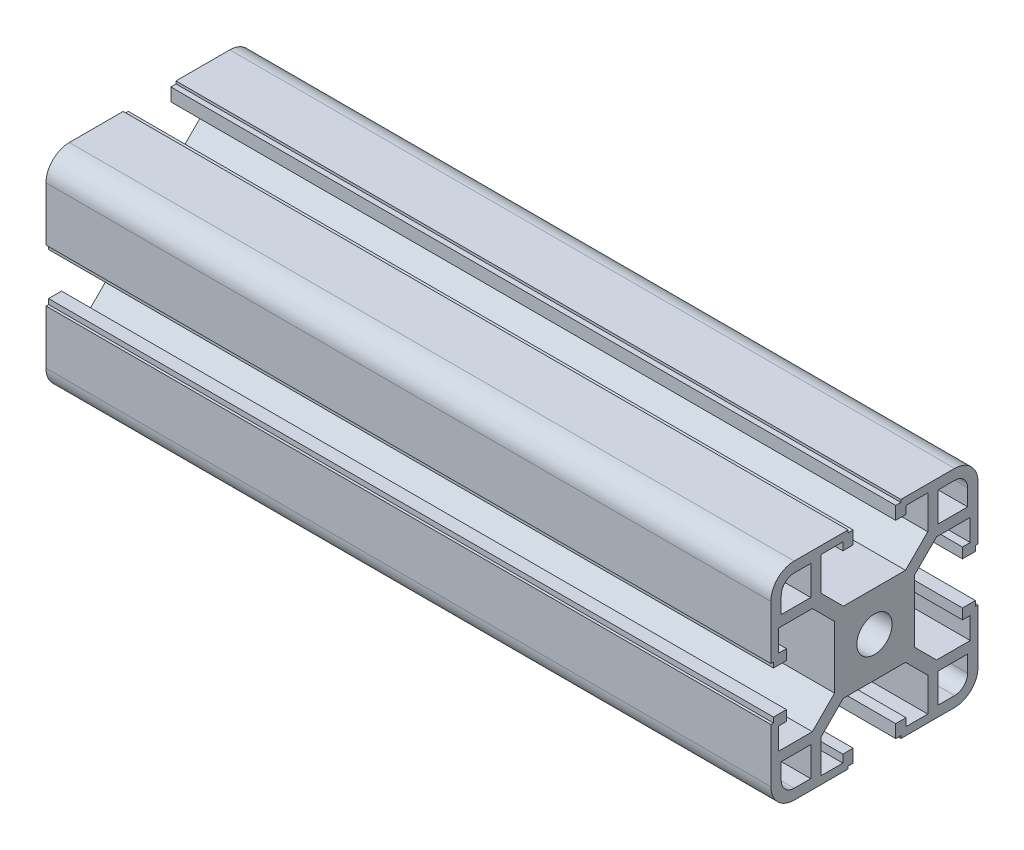
SolidWorks part; units mm, degrees
ref_plane "Front Plane" through (0, 0, 0) normal (0, 0, 1) x (1, 0, 0)
ref_plane "Top Plane" through (0, 0, 0) normal (0, 1, 0) x (1, 0, 0)
ref_plane "Right Plane" through (0, 0, 0) normal (1, 0, 0) x (0, 0, -1)
sketch "草图1" plane through (0, 0, 0) normal (0, 0, 1) x (1, 0, 0)
  line L0 (-984.975, 0) -> (-844.975, 0)
  dimension "D1" = 140
other "Aluminium profile 40 X 40B X R4.5(1)"
ref_plane "Plane1" through (-984.975, 0, 0) normal (1, 0, 0) x (0, 1, 0)
sketch "Sketch1" plane through (-984.975, 0, 0) normal (1, 0, 0) x (0, 1, 0)
  line L0 (-5.1, 20) -> (-5.1, 19.5)
  line L1 (-5.1, 19.5) -> (-4.1, 19.5)
  line L2 (-4.1, 19.5) -> (-4.1, 17)
  line L3 (-6.1, 18.5) -> (-10.3, 18.5)
  line L4 (-15.5, -20) -> (-5.1, -20)
  line L5 (-20, -15.5) -> (-20, -5.1)
  line L6 (15.5, 20) -> (5.1, 20)
  line L7 (20, 15.5) -> (20, 5.1)
  line L8 (0, 14.8756) -> (0, 0) construction
  line L9 (0, 0) -> (14.1675, 0) construction
  line L10 (-10.3, 18.5) -> (-10.3, 12)
  line L11 (-10.3, 12) -> (-6, 7.7)
  line L12 (-6, 7.7) -> (6, 7.7)
  line L13 (10.3, 12) -> (6, 7.7)
  line L14 (10.3, 18.5) -> (10.3, 12)
  line L15 (6.1, 18.5) -> (10.3, 18.5)
  line L16 (4.1, 19.5) -> (4.1, 17)
  line L17 (5.1, 19.5) -> (4.1, 19.5)
  line L18 (5.1, 20) -> (5.1, 19.5)
  line L19 (-5.1, 20) -> (-15.5, 20)
  line L20 (20, 5.1) -> (19.5, 5.1)
  line L21 (12.3, 18) -> (15.5, 18)
  line L22 (12.3, 18) -> (12.3, 12.3)
  line L23 (12.3, 12.3) -> (18, 12.3)
  line L24 (18, 15.5) -> (18, 12.3)
  line L25 (19.5, 5.1) -> (19.5, 4.1)
  line L26 (19.5, 4.1) -> (17, 4.1)
  line L27 (17, 6.1) -> (17, 4.1)
  line L28 (18.5, 6.1) -> (17, 6.1)
  line L29 (18.5, 6.1) -> (18.5, 10.3)
  line L30 (18.5, 10.3) -> (12, 10.3)
  line L31 (12, 10.3) -> (7.7, 6)
  line L32 (7.7, 6) -> (7.7, -6)
  line L33 (12, -10.3) -> (7.7, -6)
  line L34 (18.5, -10.3) -> (12, -10.3)
  line L35 (18.5, -6.1) -> (18.5, -10.3)
  line L36 (18.5, -6.1) -> (17, -6.1)
  line L37 (17, -4.1) -> (17, -6.1)
  line L38 (19.5, -4.1) -> (17, -4.1)
  line L39 (19.5, -5.1) -> (19.5, -4.1)
  line L40 (20, -5.1) -> (19.5, -5.1)
  line L41 (5.1, -20) -> (5.1, -19.5)
  line L42 (5.1, -19.5) -> (4.1, -19.5)
  line L43 (4.1, -19.5) -> (4.1, -17)
  line L44 (6.1, -17) -> (4.1, -17)
  line L45 (6.1, -18.5) -> (6.1, -17)
  line L46 (6.1, -18.5) -> (10.3, -18.5)
  line L47 (10.3, -18.5) -> (10.3, -12)
  line L48 (10.3, -12) -> (6, -7.7)
  line L49 (6, -7.7) -> (-6, -7.7)
  line L50 (-10.3, -12) -> (-6, -7.7)
  line L51 (-10.3, -18.5) -> (-10.3, -12)
  line L52 (-6.1, -18.5) -> (-10.3, -18.5)
  line L53 (-6.1, -18.5) -> (-6.1, -17)
  line L54 (-4.1, -17) -> (-6.1, -17)
  line L55 (-4.1, -19.5) -> (-4.1, -17)
  line L56 (-5.1, -19.5) -> (-4.1, -19.5)
  line L57 (-5.1, -20) -> (-5.1, -19.5)
  line L58 (-20, -5.1) -> (-19.5, -5.1)
  line L59 (5.1, -20) -> (15.5, -20)
  line L60 (-20, 5.1) -> (-20, 15.5)
  line L61 (-19.5, -5.1) -> (-19.5, -4.1)
  line L62 (-6.1, 18.5) -> (-6.1, 17)
  line L63 (-6.1, 17) -> (-4.1, 17)
  line L64 (6.1, 18.5) -> (6.1, 17)
  line L65 (4.1, 17) -> (6.1, 17)
  line L66 (-19.5, -4.1) -> (-17, -4.1)
  line L67 (-15.5, 18) -> (-12.3, 18)
  line L68 (-18, 15.5) -> (-18, 12.3)
  line L69 (-18, 12.3) -> (-12.3, 12.3)
  line L70 (-12.3, 18) -> (-12.3, 12.3)
  line L71 (-17, -6.1) -> (-17, -4.1)
  line L72 (-18.5, -6.1) -> (-17, -6.1)
  line L73 (-18.5, -6.1) -> (-18.5, -10.3)
  line L74 (-18.5, -10.3) -> (-12, -10.3)
  line L75 (-12, -10.3) -> (-7.7, -6)
  line L76 (-7.7, -6) -> (-7.7, 6)
  line L77 (-12, 10.3) -> (-7.7, 6)
  line L78 (-18.5, 10.3) -> (-12, 10.3)
  line L79 (-18.5, 6.1) -> (-18.5, 10.3)
  line L80 (-18.5, 6.1) -> (-17, 6.1)
  line L81 (-17, 4.1) -> (-17, 6.1)
  line L82 (-19.5, 4.1) -> (-17, 4.1)
  line L83 (-19.5, 5.1) -> (-19.5, 4.1)
  line L84 (-20, 5.1) -> (-19.5, 5.1)
  line L85 (20, -5.1) -> (20, -15.5)
  line L87 (-18, -12.3) -> (-12.3, -12.3)
  line L88 (-18, -12.3) -> (-18, -15.5)
  line L89 (-15.5, -18) -> (-12.3, -18)
  line L90 (-12.3, -12.3) -> (-12.3, -18)
  line L91 (12.3, -12.3) -> (18, -12.3)
  line L92 (12.3, -12.3) -> (12.3, -18)
  line L93 (12.3, -18) -> (15.5, -18)
  line L94 (18, -12.3) -> (18, -15.5)
  circle A0 centre (0, 0) radius 3.4
  arc A1 (-20, 15.5) -> (-15.5, 20) centre (-15.5, 15.5) cw
  arc A2 (20, 15.5) -> (15.5, 20) centre (15.5, 15.5) ccw
  arc A3 (-15.5, -20) -> (-20, -15.5) centre (-15.5, -15.5) cw
  arc A4 (15.5, -20) -> (20, -15.5) centre (15.5, -15.5) ccw
  arc A5 (-15.5, 18) -> (-18, 15.5) centre (-15.5, 15.5) ccw
  arc A6 (18, 15.5) -> (15.5, 18) centre (15.5, 15.5) ccw
  arc A7 (18, -15.5) -> (15.5, -18) centre (15.5, -15.5) cw
  arc A8 (-18, -15.5) -> (-15.5, -18) centre (-15.5, -15.5) ccw
  point P2 (0, 10)
  point P4 (0, 0)
  point P5 (-20, -20)
  point P6 (20, -20)
  point P7 (20, 20)
  point P8 (-20, 20)
  point P36 (-20, 20)
  point P39 (20, 20)
  point P121 (0, 0)
  dimension "D1" = 20.6
  dimension "D2" = 40
  dimension "D3" = 8.2
  dimension "D4" = 10.2
  dimension "D5" = 12.3
  dimension "D6" = 6.8
  dimension "D7" = 4.5
  dimension "D8" = 45
  dimension "D12" = 2
  dimension "D13" = 5.7
  dimension "D14" = 2
  dimension "D18" = 2.5
  dimension "D19" = 2.5
  dimension "D15" = 2.5
  dimension "D9" = 0.5
  dimension "D10" = 1.5
  dimension "D11" = 12
  dimension "D16" = 3
  dimension "D17" = 2
  dimension "D20" = 2
  dimension "D21" = 2
